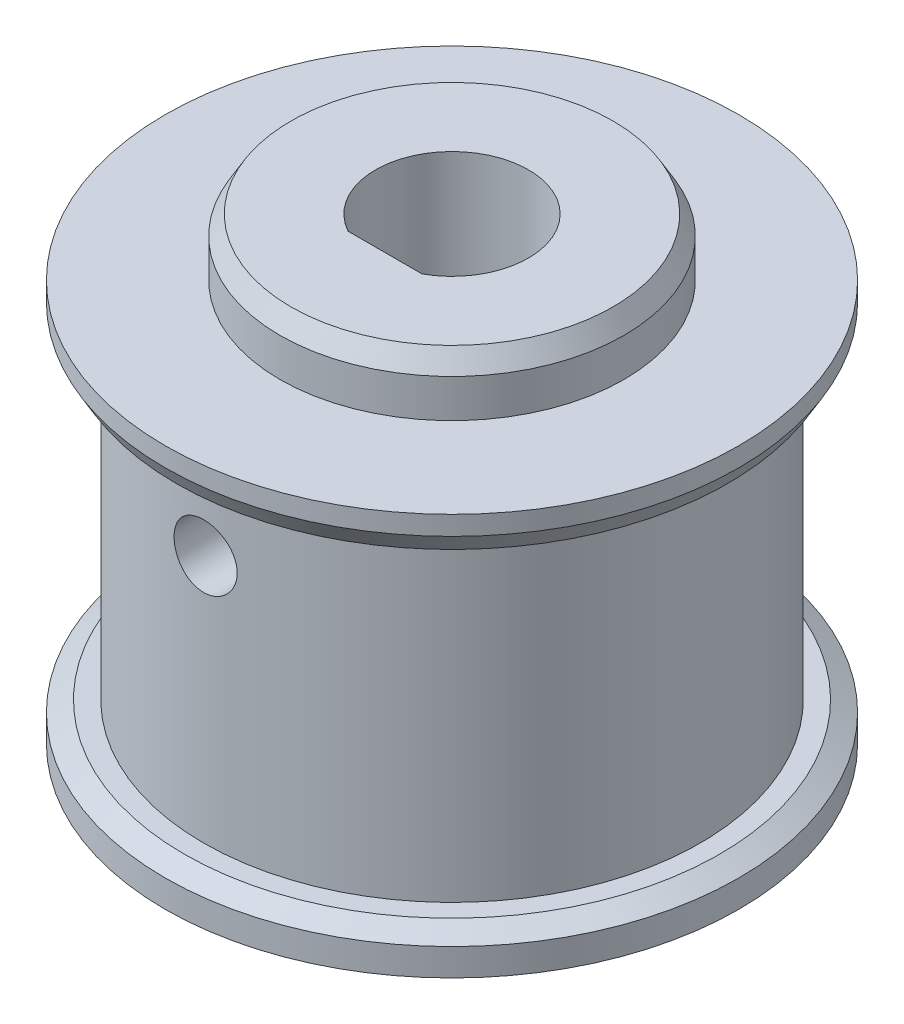
from build123d import *

# Parameters (mm, degrees)
SKETCH_5_R               = 20.566311538
CUT_EXTRUDE_1_DEPTH      = 0.5
SKETCH_6_R               = 21.52826295
CUT_EXTRUDE_2_DEPTH      = 0.5
EXTRUDE_START            = 11
SKETCH_7_R               = 8.5
SKETCH_7_R_2             = 4
EXTRUDE_1_DEPTH          = 11
SKETCH_10_R              = 15
CUT_EXTRUDE_3_DEPTH      = 15
SKETCH_11_R              = 15
SKETCH_11_R_2            = 4
EXTRUDE_2_DEPTH          = 0.5
EXTRUDE_START_2          = 0.5
SKETCH_12_R              = 15
SKETCH_12_R_2            = 4
EXTRUDE_3_DEPTH          = 0.5
EXTRUDE_START_3          = 8
SKETCH_14_R              = 7
SKETCH_14_R_2            = 4
EXTRUDE_5_DEPTH          = 8
SKETCH_17_R              = 17.215216586
CUT_EXTRUDE_4_DEPTH      = 30.849623113
SKETCH_18_R              = 9
SKETCH_18_R_2            = 4
EXTRUDE_6_DEPTH          = 8
CHAMFER_1_SIZE           = 1
CHAMFER_1_SIZE2          = 0.577350269
CHAMFER_2_SIZE           = 1
CHAMFER_2_SIZE2          = 0.577350269
CHAMFER_3_SIZE           = 0.5
EXTRUDE_8_DEPTH          = 29
SKETCH_19_W              = 1.65
SKETCH_19_H              = 15
PATTERN_CIRCULAR_1_COUNT = 2
PATTERN_CIRCULAR_1_ANGLE = 90
SKETCH_22_R              = 11.227915354
CUT_EXTRUDE_5_DEPTH      = 5
CHAMFER_4_SIZE           = 1
CHAMFER_4_SIZE2          = 0.577350269


with BuildPart() as part:
    # 草图1 → 旋转1 (revolve)
    with BuildSketch(Plane.XY, mode=Mode.PRIVATE) as revolve_1_sk:
        Polygon((4, 0), (4, 21), (15, 21), (15, 19), (12.99, 19), (12.99, 2), (15, 2), (15, 0), align=None)
    revolve(revolve_1_sk.sketch.rotate(Axis((0, 0, 0), (0, 1, 0)), 90), axis=Axis((0, 0, 0), (0, 1, 0)))

    # 草图5 → 切除-拉伸1 (cut)
    with BuildSketch(Plane.XZ):
        Circle(SKETCH_5_R)
    extrude(amount=-CUT_EXTRUDE_1_DEPTH, mode=Mode.SUBTRACT)

    # 草图6 → 切除-拉伸2 (cut)
    with BuildSketch(Plane(origin=(0, 21, 0), x_dir=(1, 0, 0), z_dir=(0, 1, 0))):
        Circle(SKETCH_6_R)
    extrude(amount=-CUT_EXTRUDE_2_DEPTH, mode=Mode.SUBTRACT)

    # 草图7 → 凸台-拉伸1 (add)
    with BuildSketch(Plane(origin=(0, 20.5, 0), x_dir=(1, 0, 0), z_dir=(0, 1, 0)).offset(EXTRUDE_START)):
        with Locations(Location((0, 0, 0), (0, 0, 270))):
            Circle(SKETCH_7_R)
        with Locations(Location((0, 0, 0), (0, 0, 90))):
            Circle(SKETCH_7_R_2, mode=Mode.SUBTRACT)
    extrude(amount=-EXTRUDE_1_DEPTH)

    # 草图10 → 切除-拉伸3 (cut)
    with BuildSketch(Plane(origin=(0, 20.5, 0), x_dir=(1, 0, 0), z_dir=(0, 1, 0))):
        with Locations(Location((0, 0, 0), (0, 0, 90))):
            Circle(SKETCH_10_R)
    extrude(amount=CUT_EXTRUDE_3_DEPTH, mode=Mode.SUBTRACT)

    # 草图11 → 凸台-拉伸2 (add)
    with BuildSketch(Plane(origin=(0, 20.5, 0), x_dir=(1, 0, 0), z_dir=(0, 1, 0))):
        with Locations(Location((0, 0, 0), (0, 0, 90))):
            Circle(SKETCH_11_R)
        with Locations(Location((0, 0, 0), (0, 0, 90))):
            Circle(SKETCH_11_R_2, mode=Mode.SUBTRACT)
    extrude(amount=EXTRUDE_2_DEPTH)

    # 草图12 → 凸台-拉伸3 (add)
    with BuildSketch(Plane.XZ.offset(-0.5).offset(EXTRUDE_START_2)):
        with Locations(Location((0, 0, 0), (0, 0, 270))):
            Circle(SKETCH_12_R)
        with Locations(Location((0, 0, 0), (0, 0, 270))):
            Circle(SKETCH_12_R_2, mode=Mode.SUBTRACT)
    extrude(amount=-EXTRUDE_3_DEPTH)

    # 草图14 → 凸台-拉伸5 (add)
    with BuildSketch(Plane(origin=(0, 21, 0), x_dir=(1, 0, 0), z_dir=(0, 1, 0)).offset(EXTRUDE_START_3)):
        with Locations(Location((0, 0, 0), (0, 0, 270))):
            Circle(SKETCH_14_R)
        with Locations(Location((0, 0, 0), (0, 0, 90))):
            Circle(SKETCH_14_R_2, mode=Mode.SUBTRACT)
    extrude(amount=-EXTRUDE_5_DEPTH)

    # 草图17 → 切除-拉伸4 (cut, through all)
    with BuildSketch(Plane(origin=(0, 21, 0), x_dir=(1, 0, 0), z_dir=(0, 1, 0))):
        Circle(SKETCH_17_R)
    extrude(amount=CUT_EXTRUDE_4_DEPTH, mode=Mode.SUBTRACT)

    # 草图18 → 凸台-拉伸6 (add)
    with BuildSketch(Plane(origin=(0, 21, 0), x_dir=(1, 0, 0), z_dir=(0, 1, 0)).offset(EXTRUDE_START_3)):
        with Locations(Location((0, 0, 0), (0, 0, 270))):
            Circle(SKETCH_18_R)
        with Locations(Location((0, 0, 0), (0, 0, 90))):
            Circle(SKETCH_18_R_2, mode=Mode.SUBTRACT)
    extrude(amount=-EXTRUDE_6_DEPTH)

    # 倒角1
    chamfer_1_edges = [part.edges().sort_by_distance(p)[0] for p in [
        (0, 19, 15),
    ]]
    chamfer_1_side = [part.faces().sort_by_distance(p)[0] for p in [
        (0, 20, 15),
    ]]
    chamfer(chamfer_1_edges, length=CHAMFER_1_SIZE, length2=CHAMFER_1_SIZE2, reference=chamfer_1_side[0])

    # 倒角2
    chamfer_2_edges = [part.edges().sort_by_distance(p)[0] for p in [
        (0, 2, 15),
    ]]
    chamfer_2_side = [part.faces().sort_by_distance(p)[0] for p in [
        (0, 2, 13.414264069),
    ]]
    chamfer(chamfer_2_edges, length=CHAMFER_2_SIZE, length2=CHAMFER_2_SIZE2, reference=chamfer_2_side[0])

    # 倒角3
    chamfer_3_edges = [part.edges().sort_by_distance(p)[0] for p in [
        (0, 29, -9),
    ]]
    chamfer(chamfer_3_edges, length=CHAMFER_3_SIZE)

    # 草图21 → 凸台-拉伸8 (add, through all)
    with BuildSketch(Plane(origin=(0, 29, 0), x_dir=(1, 0, 0), z_dir=(0, 1, 0))):
        with BuildLine():
            Line((-1.936491673, -3.5), (1.936491673, -3.5))
            ThreePointArc((1.936491673, -3.5), (0, -4), (-1.936491673, -3.5))
        make_face()
    extrude(amount=-EXTRUDE_8_DEPTH)

    # 草图19 → M4 螺纹孔1 (revolve, cut)
    with BuildSketch(Plane(origin=(0, 15, 0), x_dir=(0, 1, 0), z_dir=(1, 0, 0))):
        with Locations((0.825, 7.5)):
            Rectangle(SKETCH_19_W, SKETCH_19_H)
    hole_wizard_m4_1 = revolve(axis=Axis((0, 15, -6.35), (0, 0, 1)), mode=Mode.SUBTRACT)

    # 阵列(圆周)1: M4 螺纹孔1 ×2 about axis
    pattern_circular_1_axis = Axis((0, 0, 0), (0, -1, 0))
    for i in range(1, PATTERN_CIRCULAR_1_COUNT):
        add(hole_wizard_m4_1.rotate(pattern_circular_1_axis, i * PATTERN_CIRCULAR_1_ANGLE / (PATTERN_CIRCULAR_1_COUNT - 1)), mode=Mode.SUBTRACT)

    # 草图22 → 切除-拉伸5 (cut)
    with BuildSketch(Plane(origin=(0, 29, 0), x_dir=(1, 0, 0), z_dir=(0, 1, 0))):
        Circle(SKETCH_22_R)
    extrude(amount=-CUT_EXTRUDE_5_DEPTH, mode=Mode.SUBTRACT)

    # 倒角4
    chamfer_4_edges = [part.edges().sort_by_distance(p)[0] for p in [
        (0, 24, -9),
    ]]
    chamfer_4_side = [part.faces().sort_by_distance(p)[0] for p in [
        (0, 22.5, -9),
    ]]
    chamfer(chamfer_4_edges, length=CHAMFER_4_SIZE, length2=CHAMFER_4_SIZE2, reference=chamfer_4_side[0])


solid = part.part
